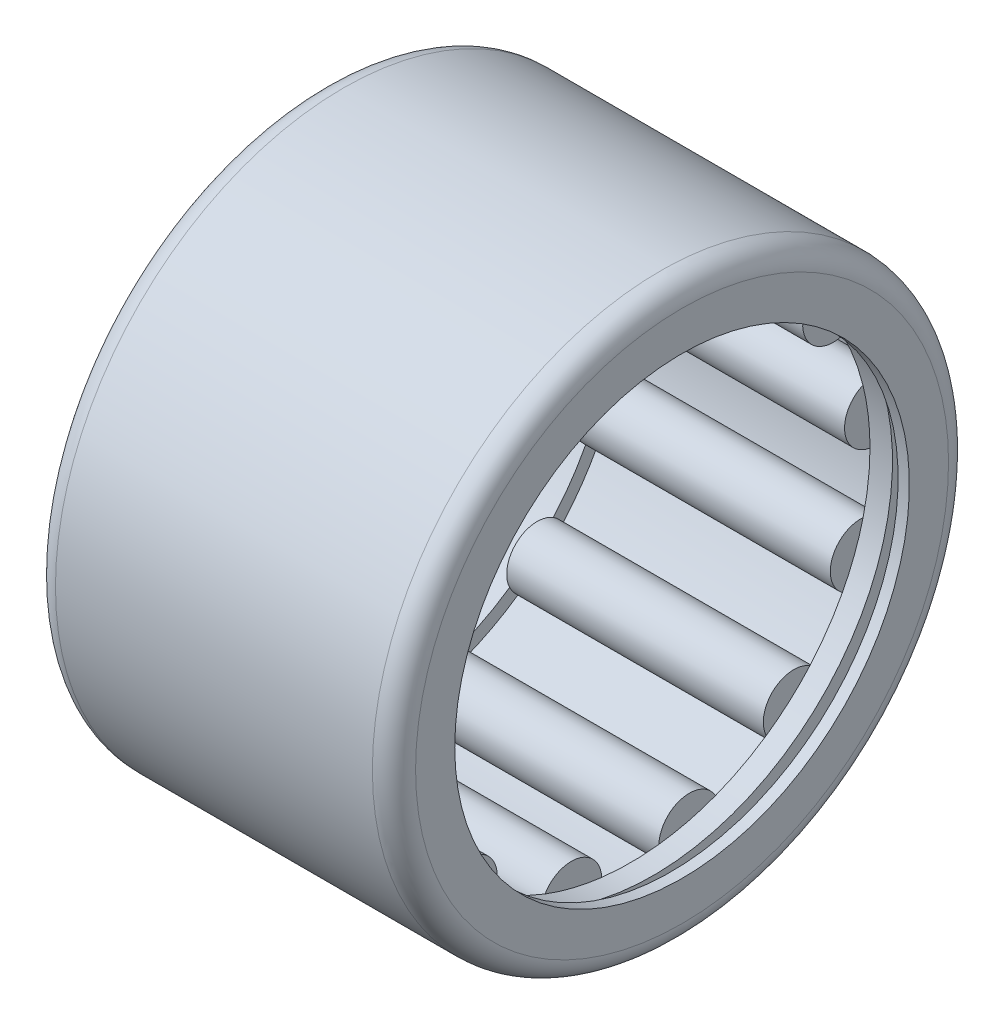
from build123d import *

# Parameters (mm, degrees)
SKETCH5_W         = 0.625
SKETCH5_H         = 0.375
SKETCH6_W         = 0.4125
SKETCH6_H         = 0.2375
CIRPATTERN3_COUNT = 13
CIRPATTERN2_COUNT = 13
FILLET1_R         = 0.6


with BuildPart() as part:
    # Sketch5 → Base-Revolve2 (revolve)
    with BuildSketch(Plane.XY, mode=Mode.PRIVATE) as base_revolve2_sk:
        with Locations((1.125, 6.84375)):
            Rectangle(SKETCH5_W, SKETCH5_H)
    base_revolve2 = revolve(base_revolve2_sk.sketch.rotate(Axis((0, 0, 0), (1, 0, 0)), 90), axis=Axis((0, 0, 0), (1, 0, 0)))

    # Sketch6 → Cut-Revolve1 (revolve, cut)
    with BuildSketch(Plane.XY):
        with Locations((1.28125, 6.725)):
            Rectangle(SKETCH6_W, SKETCH6_H)
    cut_revolve1 = revolve(axis=Axis((-4.603138189, 6.84375, 0), (1, 0, 0)), mode=Mode.SUBTRACT)

    # CirPattern3: Cut-Revolve1 ×13 about axis
    cirpattern3_axis = Axis((0, 0, 0), (1, 0, 0))
    for i in range(1, CIRPATTERN3_COUNT):
        add(cut_revolve1.rotate(cirpattern3_axis, i * 360 / CIRPATTERN3_COUNT), mode=Mode.SUBTRACT)

    # Sketch3 → Base-Revolve (revolve)
    with BuildSketch(Plane.XY, mode=Mode.PRIVATE) as base_revolve_sk:
        Polygon((1.4375, 7.6885), (8.5625, 7.6885), (8.5625, 7.03125), (8.875, 7.03125), (8.875, 6.84375), (1.125, 6.84375), (1.125, 7.03125), (1.4375, 7.03125), align=None)
    base_revolve = revolve(base_revolve_sk.sketch.rotate(Axis((-4.603138189, 6.84375, 0), (1, 0, 0)), 90), axis=Axis((-4.603138189, 6.84375, 0), (1, 0, 0)))

    # Sketch2 → Boss-Revolve2 (revolve)
    with BuildSketch(Plane.XY, mode=Mode.PRIVATE) as boss_revolve2_sk:
        Polygon((9.6875, 6.3125), (10, 6.3125), (10, 8), (0, 8), (0, 6.3125), (0.3125, 6.3125), (0.3125, 7.6875), (9.6875, 7.6875), align=None)
    revolve(boss_revolve2_sk.sketch.rotate(Axis((0, 0, 0), (1, 0, 0)), 90), axis=Axis((0, 0, 0), (1, 0, 0)))

    # Mirror1: Base-Revolve2 across plane
    add(base_revolve2.mirror(Plane.ZY.offset(-5)))

    # CirPattern2: Base-Revolve ×13 about axis
    cirpattern2_axis = Axis((0, 0, 0), (1, 0, 0))
    for i in range(1, CIRPATTERN2_COUNT):
        add(base_revolve.rotate(cirpattern2_axis, i * 360 / CIRPATTERN2_COUNT))

    # Fillet1
    fillet1_edges = [part.edges().sort_by_distance(p)[0] for p in [
        (0, 0, -8),
        (10, 0, -8),
    ]]
    fillet(fillet1_edges, radius=FILLET1_R)

    # Mirror2: Base-Revolve across plane
    add(base_revolve.mirror(Plane.ZY.offset(-5)))


solid = part.part
